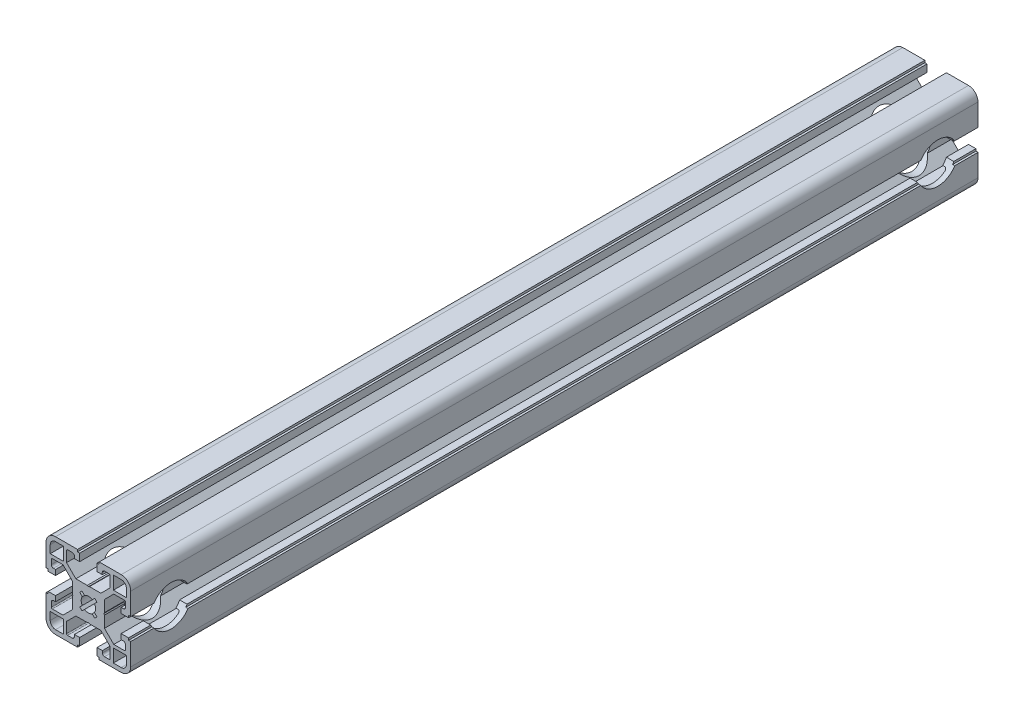
SolidWorks part; units mm, degrees
material "6061 GB/T6892-2006"
ref_plane "前视" through (0, 0, 0) normal (0, 0, 1) x (1, 0, 0)
ref_plane "上视" through (0, 0, 0) normal (0, 1, 0) x (1, 0, 0)
ref_plane "右视" through (0, 0, 0) normal (1, 0, 0) x (0, 0, -1)
sketch "草图1" plane through (0, 0, 0) normal (0, 0, 1) x (1, 0, 0)
  line L0 (-18.9995, -4.1003) -> (-18.9995, -5.1003)
  line L1 (-18.9995, -5.1003) -> (-19.9995, -5.1003)
  line L2 (-19.9995, -5.1003) -> (-19.9995, -15.5003)
  line L3 (-15.4995, -20.0003) -> (-5.0995, -20.0003)
  line L4 (-5.0995, -20.0003) -> (-5.0995, -19.0003)
  line L5 (-5.0995, -19.0003) -> (-4.0995, -19.0003)
  line L6 (-4.0995, -19.0003) -> (-4.0995, -15.5003)
  line L7 (-4.0995, -15.5003) -> (-6.5995, -15.5003)
  line L8 (-6.5995, -15.5003) -> (-6.5995, -16.5003)
  line L9 (-7.5995, -17.5003) -> (-9.7995, -17.5003)
  line L10 (-10.2995, -17.0003) -> (-10.2995, -11.9973)
  line L11 (-10.2995, -11.9973) -> (-5.9025, -7.6003)
  line L12 (-5.9025, -7.6003) -> (-0.5195, -7.6003)
  line L13 (-0.5195, -7.6003) -> (0.0005, -7.3003)
  line L14 (0.0005, -7.3003) -> (0.5195, -7.6003)
  line L15 (0.5195, -7.6003) -> (5.9035, -7.6003)
  line L16 (5.9035, -7.6003) -> (10.3005, -11.9973)
  line L17 (10.3005, -11.9973) -> (10.3005, -17.0003)
  line L18 (9.8005, -17.5003) -> (7.6005, -17.5003)
  line L19 (6.6005, -16.5003) -> (6.6005, -15.5003)
  line L20 (6.6005, -15.5003) -> (4.1005, -15.5003)
  line L21 (4.1005, -15.5003) -> (4.1005, -19.0003)
  line L22 (4.1005, -19.0003) -> (5.1005, -19.0003)
  line L23 (5.1005, -19.0003) -> (5.1005, -20.0003)
  line L24 (5.1005, -20.0003) -> (15.5005, -20.0003)
  line L25 (20.0005, -15.5003) -> (20.0005, -5.1003)
  line L26 (20.0005, -5.1003) -> (19.0005, -5.1003)
  line L27 (19.0005, -5.1003) -> (19.0005, -4.1003)
  line L28 (19.0005, -4.1003) -> (15.5005, -4.1003)
  line L29 (15.5005, -4.1003) -> (15.5005, -6.6003)
  line L30 (15.5005, -6.6003) -> (16.5005, -6.6003)
  line L31 (17.5005, -7.6003) -> (17.5005, -9.8003)
  line L32 (17.0005, -10.3003) -> (11.9975, -10.3003)
  line L33 (11.9975, -10.3003) -> (7.6005, -5.9033)
  line L34 (7.6005, -5.9033) -> (7.6005, -0.5203)
  line L35 (7.6005, -0.5203) -> (7.3005, -0.0003)
  line L36 (7.3005, -0.0003) -> (7.6005, 0.5197)
  line L37 (7.6005, 0.5197) -> (7.6005, 5.9027)
  line L38 (7.6005, 5.9027) -> (11.9975, 10.2997)
  line L39 (11.9975, 10.2997) -> (17.0005, 10.2997)
  line L40 (17.5005, 9.7997) -> (17.5005, 7.5997)
  line L41 (16.5005, 6.5997) -> (15.5005, 6.5997)
  line L42 (15.5005, 6.5997) -> (15.5005, 4.0997)
  line L43 (15.5005, 4.0997) -> (19.0005, 4.0997)
  line L44 (19.0005, 4.0997) -> (19.0005, 5.0997)
  line L45 (19.0005, 5.0997) -> (20.0005, 5.0997)
  line L46 (20.0005, 5.0997) -> (20.0005, 15.4997)
  line L47 (15.5005, 19.9997) -> (5.1005, 19.9997)
  line L48 (5.1005, 19.9997) -> (5.1005, 18.9997)
  line L49 (5.1005, 18.9997) -> (4.1005, 18.9997)
  line L50 (4.1005, 18.9997) -> (4.1005, 15.4997)
  line L51 (4.1005, 15.4997) -> (6.6005, 15.4997)
  line L52 (7.6005, 17.4997) -> (9.8005, 17.4997)
  line L53 (10.3005, 16.9997) -> (10.3005, 11.9967)
  line L54 (10.3005, 11.9967) -> (5.9035, 7.5997)
  line L55 (5.9035, 7.5997) -> (0.5195, 7.5997)
  line L56 (0.5195, 7.5997) -> (0.0005, 7.2997)
  line L57 (0.0005, 7.2997) -> (-0.5195, 7.5997)
  line L58 (-0.5195, 7.5997) -> (-5.9025, 7.5997)
  line L59 (-5.9025, 7.5997) -> (-10.2995, 11.9967)
  line L60 (-10.2995, 11.9967) -> (-10.2995, 16.9997)
  line L61 (-9.7995, 17.4997) -> (-7.5995, 17.4997)
  line L62 (-6.5995, 16.4997) -> (-6.5995, 15.4997)
  line L63 (-6.5995, 15.4997) -> (-4.0995, 15.4997)
  line L64 (-4.0995, 15.4997) -> (-4.0995, 18.9997)
  line L65 (-4.0995, 18.9997) -> (-5.0995, 18.9997)
  line L66 (-5.0995, 18.9997) -> (-5.0995, 19.9997)
  line L67 (-5.0995, 19.9997) -> (-15.4995, 19.9997)
  line L68 (-19.9995, 15.4997) -> (-19.9995, 5.0997)
  line L69 (-19.9995, 5.0997) -> (-18.9995, 5.0997)
  line L70 (-18.9995, 5.0997) -> (-18.9995, 4.0997)
  line L71 (-18.9995, 4.0997) -> (-15.4995, 4.0997)
  line L72 (-15.4995, 4.0997) -> (-15.4995, 6.5997)
  line L73 (-15.4995, 6.5997) -> (-16.4995, 6.5997)
  line L74 (-17.4995, 7.5997) -> (-17.4995, 9.7997)
  line L75 (-16.9995, 10.2997) -> (-11.9965, 10.2997)
  line L76 (-11.9965, 10.2997) -> (-7.5995, 5.9027)
  line L77 (-7.5995, 5.9027) -> (-7.5995, 0.5197)
  line L78 (-7.5995, 0.5197) -> (-7.2995, -0.0003)
  line L79 (-7.2995, -0.0003) -> (-7.5995, -0.5203)
  line L80 (-7.5995, -0.5203) -> (-7.5995, -5.9033)
  line L81 (-7.5995, -5.9033) -> (-11.9965, -10.3003)
  line L82 (-11.9965, -10.3003) -> (-16.9995, -10.3003)
  line L83 (-17.4995, -9.8003) -> (-17.4995, -7.6003)
  line L84 (-16.4995, -6.6003) -> (-15.4995, -6.6003)
  line L85 (-15.4995, -6.6003) -> (-15.4995, -4.1003)
  line L86 (-15.4995, -4.1003) -> (-18.9995, -4.1003)
  line L87 (15.5005, -18.0003) -> (11.8005, -18.0003)
  line L88 (11.8005, -18.0003) -> (11.8005, -11.8003)
  line L89 (11.8005, -11.8003) -> (18.0005, -11.8003)
  line L90 (18.0005, -11.8003) -> (18.0005, -15.5003)
  line L91 (18.0005, 11.7997) -> (11.8005, 11.7997)
  line L92 (11.8005, 11.7997) -> (11.8005, 17.9997)
  line L93 (11.8005, 17.9997) -> (15.5005, 17.9997)
  line L94 (18.0005, 15.4997) -> (18.0005, 11.7997)
  line L95 (-1.8145, -2.8753) -> (-3.0044, -4.0665)
  line L96 (-3.0044, -4.0665) -> (-4.0656, -3.0052)
  line L97 (-4.0656, -3.0052) -> (-2.8745, -1.8153)
  line L98 (-2.8745, 1.8147) -> (-4.0644, 3.0058)
  line L99 (-4.0644, 3.0058) -> (-3.0044, 4.0658)
  line L100 (-3.0044, 4.0658) -> (-1.8145, 2.8747)
  line L101 (1.8145, 2.8747) -> (3.0055, 4.0657)
  line L102 (3.0055, 4.0657) -> (4.0666, 3.0045)
  line L103 (4.0666, 3.0045) -> (2.8755, 1.8147)
  line L104 (2.8755, -1.8153) -> (4.0666, -3.0052)
  line L105 (4.0666, -3.0052) -> (3.0055, -4.0663)
  line L106 (3.0055, -4.0663) -> (1.8145, -2.8753)
  line L107 (-17.9995, -15.5003) -> (-17.9995, -11.8003)
  line L108 (-17.9995, -11.8003) -> (-11.7995, -11.8003)
  line L109 (-11.7995, -11.8003) -> (-11.7995, -18.0003)
  line L110 (-11.7995, -18.0003) -> (-15.4995, -18.0003)
  line L111 (-11.7995, 17.9997) -> (-11.7995, 11.7997)
  line L112 (-11.7995, 11.7997) -> (-17.9995, 11.7997)
  line L113 (-17.9995, 11.7997) -> (-17.9995, 15.4997)
  line L114 (-15.4995, 17.9997) -> (-11.7995, 17.9997)
  arc A0 (-19.9995, -15.5003) -> (-15.4995, -20.0003) centre (-15.4995, -15.5003) ccw
  arc A1 (-6.5995, -16.5003) -> (-7.5995, -17.5003) centre (-7.5995, -16.5003) cw
  arc A2 (-9.7995, -17.5003) -> (-10.2995, -17.0003) centre (-9.7995, -17.0003) cw
  arc A3 (10.3005, -17.0003) -> (9.8005, -17.5003) centre (9.8005, -17.0003) cw
  arc A4 (7.6005, -17.5003) -> (6.6005, -16.5003) centre (7.6005, -16.5003) cw
  arc A5 (15.5005, -20.0003) -> (20.0005, -15.5003) centre (15.5005, -15.5003) ccw
  arc A6 (16.5005, -6.6003) -> (17.5005, -7.6003) centre (16.5005, -7.6003) cw
  arc A7 (17.5005, -9.8003) -> (17.0005, -10.3003) centre (17.0005, -9.8003) cw
  arc A8 (17.0005, 10.2997) -> (17.5005, 9.7997) centre (17.0005, 9.7997) cw
  arc A9 (17.5005, 7.5997) -> (16.5005, 6.5997) centre (16.5005, 7.5997) cw
  arc A10 (20.0005, 15.4997) -> (15.5005, 19.9997) centre (15.5005, 15.4997) ccw
  arc A11 (6.6005, 15.4997) -> (6.6005, 16.4997) centre (7.1003, 15.9997) cw
  arc A12 (6.6005, 16.4997) -> (7.6005, 17.4997) centre (7.6005, 16.4997) cw
  arc A13 (9.8005, 17.4997) -> (10.3005, 16.9997) centre (9.8005, 16.9997) cw
  arc A14 (-10.2995, 16.9997) -> (-9.7995, 17.4997) centre (-9.7995, 16.9997) cw
  arc A15 (-7.5995, 17.4997) -> (-6.5995, 16.4997) centre (-7.5995, 16.4997) cw
  arc A16 (-15.4995, 19.9997) -> (-19.9995, 15.4997) centre (-15.4995, 15.4997) ccw
  arc A17 (-16.4995, 6.5997) -> (-17.4995, 7.5997) centre (-16.4995, 7.5997) cw
  arc A18 (-17.4995, 9.7997) -> (-16.9995, 10.2997) centre (-16.9995, 9.7997) cw
  arc A19 (-16.9995, -10.3003) -> (-17.4995, -9.8003) centre (-16.9995, -9.8003) cw
  arc A20 (-17.4995, -7.6003) -> (-16.4995, -6.6003) centre (-16.4995, -7.6003) cw
  arc A21 (18.0005, -15.5003) -> (15.5005, -18.0003) centre (15.5005, -15.5003) cw
  arc A22 (15.5005, 17.9997) -> (18.0005, 15.4997) centre (15.5005, 15.4997) cw
  arc A23 (-2.8745, -1.8153) -> (-2.8745, 1.8147) centre (0.0005, -0.0003) cw
  arc A24 (-1.8145, 2.8747) -> (1.8145, 2.8747) centre (0, -0.0007) cw
  arc A25 (2.8755, 1.8147) -> (2.8755, -1.8153) centre (0.0005, -0.0003) cw
  arc A26 (1.8145, -2.8753) -> (-1.8145, -2.8753) centre (0, 0) cw
  arc A27 (-15.4995, -18.0003) -> (-17.9995, -15.5003) centre (-15.4995, -15.5003) cw
  arc A28 (-17.9995, 15.4997) -> (-15.4995, 17.9997) centre (-15.4995, 15.4997) cw
extrude "凸台-拉伸1" add sketch "草图1" against normal blind 400
hole_wizard "Ø19.0 (19) 直径孔1" positions "草图2" profile "草图3" hole size "Ø19.0" standard "GB" end condition through all
sketch "草图2" plane through (20.0005, 0, 0) normal (1, 0, 0) x (0, 0, -1)
  line L0 (400, -0.0003) -> (0, -0.0003) construction
  line L1 (400, -0.0003) -> (0, -0.0003) construction
  point P0 (381, -0.0003)
  point P6 (19, -0.0003)
  dimension "D1" = 19
  dimension "D2" = 19
sketch "草图3" plane through (20.0005, -0.0003, -381) normal (0, 1, 0) x (0, 0, -1)
  line L0 (0, 0) -> (0, 40)
  line L1 (0, 40) -> (9.5, 40)
  line L2 (9.5, 40) -> (9.5, 0)
  line L5 (9.5, 0) -> (0, 0)
  line L11 (0, -6.35) -> (0, 107.95) construction
  dimension "通孔孔直径" = 19
  dimension "通孔孔深度" = 40
